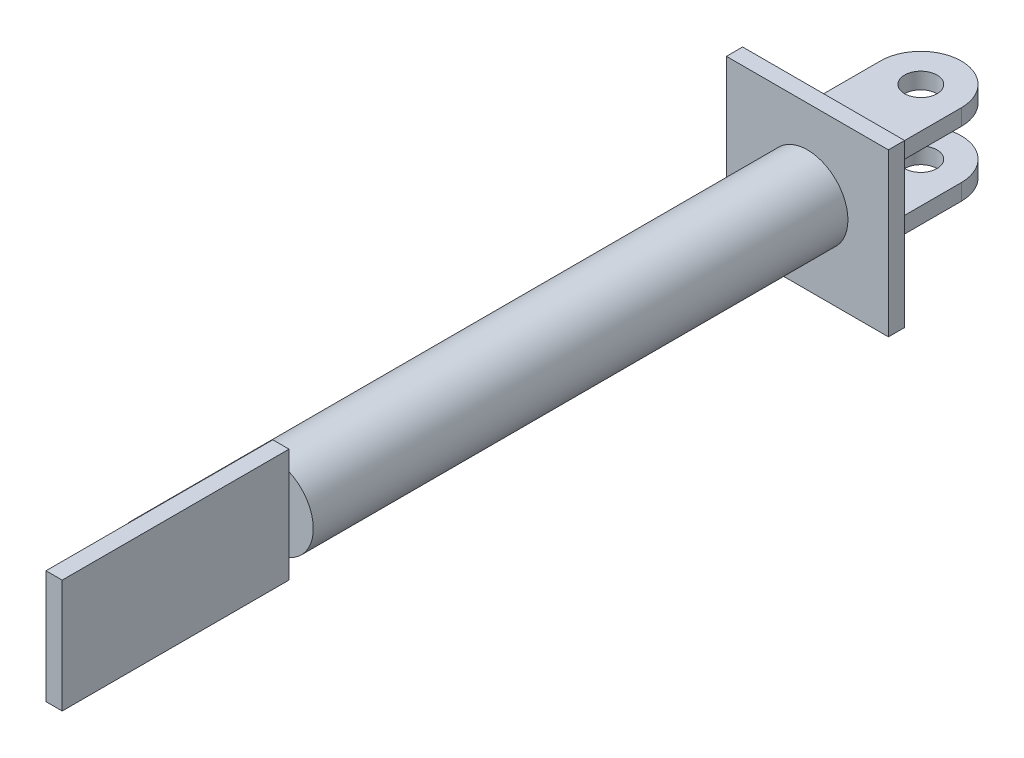
from build123d import *

# Parameters (mm, degrees)
SKETCH1_W           = 100
SKETCH1_H           = 100
BOSS_EXTRUDE1_DEPTH = 5
SKETCH2_R           = 10
BOSS_EXTRUDE2_DEPTH = 25
SKETCH3_W           = 50
SKETCH3_H           = 30
CUT_EXTRUDE1_DEPTH  = 130
SKETCH4_R           = 25
BOSS_EXTRUDE3_DEPTH = 400
CUT_EXTRUDE2_START  = -70
CUT_EXTRUDE2_DEPTH  = 70
SKETCH7_W           = 140
SKETCH7_H           = 70
BOSS_EXTRUDE4_DEPTH = 10


with BuildPart() as part:
    # Sketch1 → Boss-Extrude1 (new, symmetric)
    with BuildSketch(Plane.XY):
        Rectangle(SKETCH1_W, SKETCH1_H)
    extrude(amount=BOSS_EXTRUDE1_DEPTH, both=True)

    # Sketch2 → Boss-Extrude2 (add, symmetric)
    with BuildSketch(Plane(origin=(0, 0, 0), x_dir=(1, 0, 0), z_dir=(0, 1, 0))):
        with BuildLine():
            Line((-25, 5), (25, 5))
            Line((25, 5), (25, 65))
            ThreePointArc((25, 65), (0, 90), (-25, 65))
            Line((-25, 65), (-25, 5))
        make_face()
        with Locations(Location((0, 65, 0), (0, 0, 270))):
            Circle(SKETCH2_R, mode=Mode.SUBTRACT)
    extrude(amount=BOSS_EXTRUDE2_DEPTH, both=True)

    # Sketch3 → Cut-Extrude1 (cut)
    with BuildSketch(Plane(origin=(0, 0, -5), x_dir=(-1, 0, 0), z_dir=(0, 0, -1))):
        Rectangle(SKETCH3_W, SKETCH3_H)
    extrude(amount=CUT_EXTRUDE1_DEPTH, mode=Mode.SUBTRACT)

    # Sketch4 → Boss-Extrude3 (add)
    with BuildSketch(Plane.XY.offset(5)):
        with Locations(Location((0, 0, 0), (0, 0, 180))):
            Circle(SKETCH4_R)
    extrude(amount=BOSS_EXTRUDE3_DEPTH)

    # Sketch5 → Cut-Extrude2 (cut)
    with BuildSketch(Plane.XY.offset(405).offset(CUT_EXTRUDE2_START)):
        with BuildLine():
            Line((0, 25), (0, -25))
            ThreePointArc((0, -25), (25, 0), (0, 25))
        make_face()
    extrude(amount=CUT_EXTRUDE2_DEPTH, mode=Mode.SUBTRACT)

    # Sketch7 → Boss-Extrude4 (add)
    with BuildSketch(Plane(origin=(0, 0, 0), x_dir=(0, 0, -1), z_dir=(1, 0, 0))):
        with Locations((-405, 0)):
            Rectangle(SKETCH7_W, SKETCH7_H)
    extrude(amount=BOSS_EXTRUDE4_DEPTH)


solid = part.part
